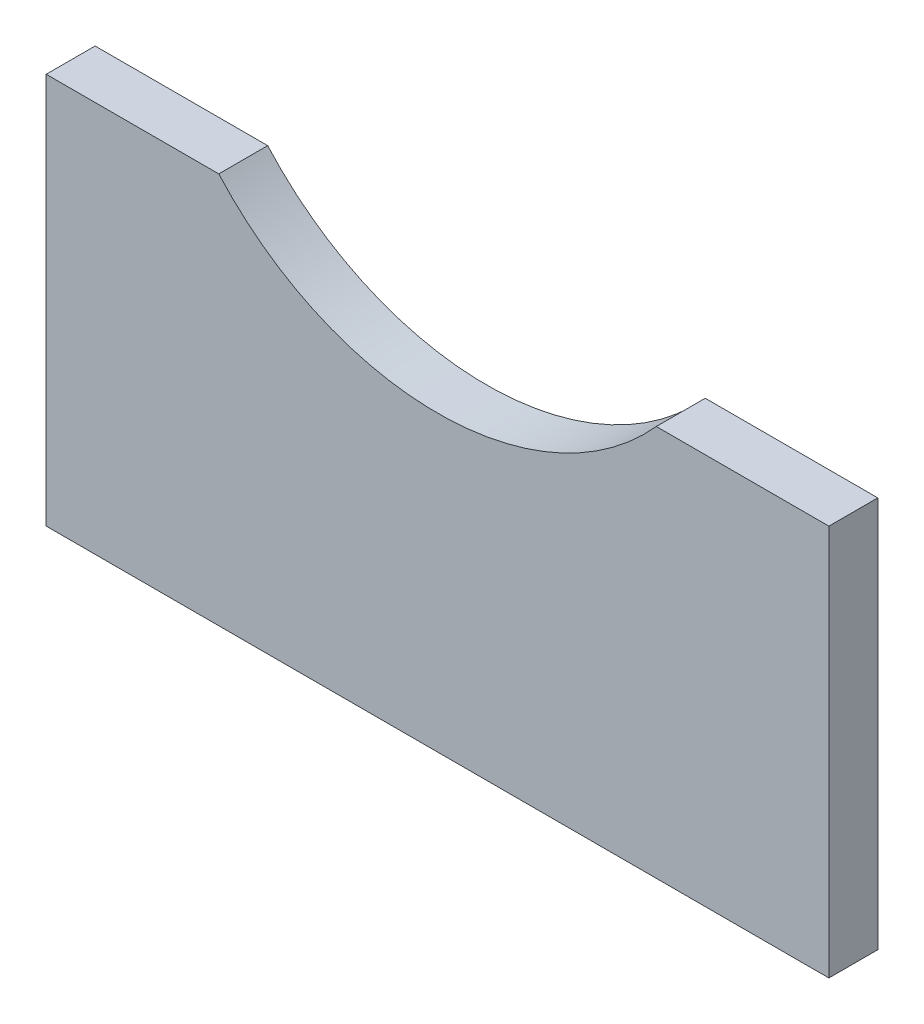
from build123d import *

# Parameters (mm, degrees)
BOSS_EXTRUDE1_DEPTH = 9.525


with BuildPart() as part:
    # Sketch1 → Boss-Extrude1 (new body)
    with BuildSketch(Plane.XY.offset(133.35)):
        with BuildLine():
            Line((-76.2, -38.1), (-42.597094971, -38.1))
            ThreePointArc((-42.597094971, -38.1), (0, -57.15), (42.597094971, -38.1))
            Line((42.597094971, -38.1), (76.2, -38.1))
            Line((76.2, -38.1), (76.2, -114.3))
            Line((76.2, -114.3), (-76.2, -114.3))
            Line((-76.2, -114.3), (-76.2, -38.1))
        make_face()
    extrude(amount=-BOSS_EXTRUDE1_DEPTH)


solid = part.part
